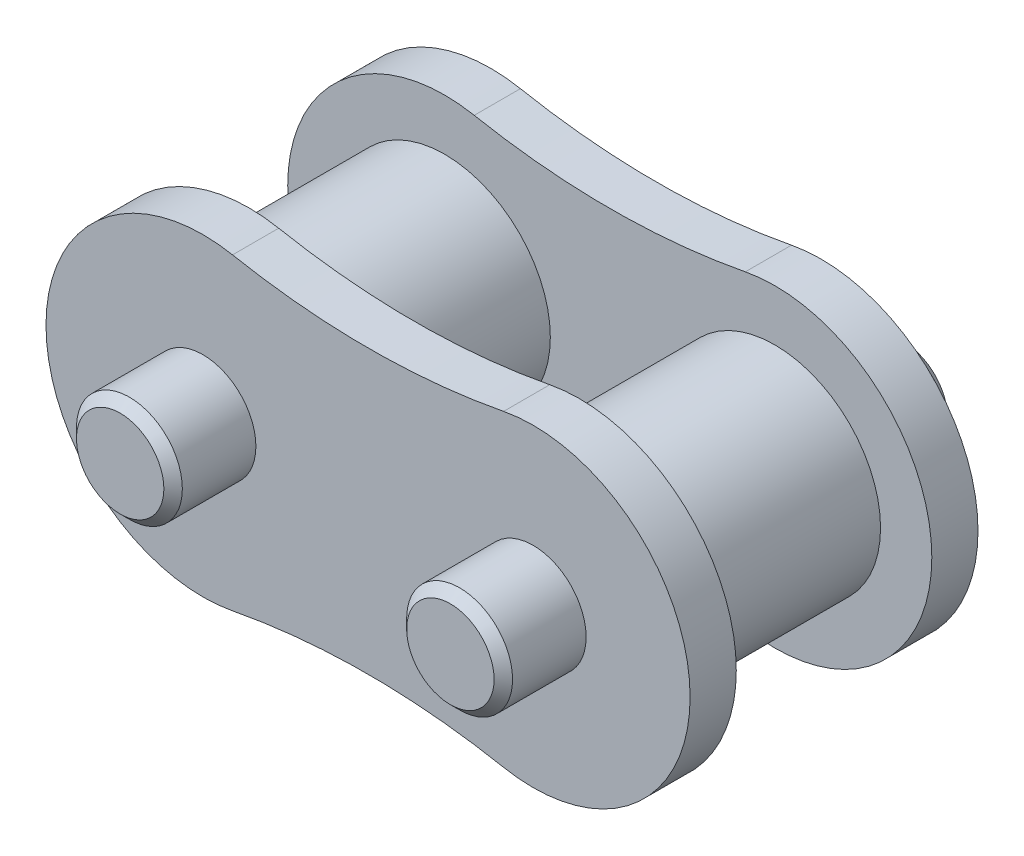
from build123d import *

# Parameters (mm, degrees)
SKETCH_2_R        = 5.08
EXTRUDE_1_DEPTH   = 4.7
EXTRUDE_1_2_DEPTH = 4.7
EXTRUDE_2_DEPTH   = 2.22
SKETCH_4_R        = 2.545
EXTRUDE_3_DEPTH   = 10.9
CHAMFER_1_SIZE    = 0.444


with BuildPart() as part:
    # 草图2 → 拉伸1 (new, symmetric)
    with BuildSketch(Plane.XY):
        with Locations((7.9375, 0)):
            Circle(SKETCH_2_R)
    extrude(amount=EXTRUDE_1_DEPTH, both=True)



with BuildPart() as body_2:
    # 草图2 → Extrude 1 2 (new, symmetric)
    with BuildSketch(Plane.XY):
        with Locations((-7.9375, 0)):
            Circle(SKETCH_2_R)
    extrude(amount=EXTRUDE_1_2_DEPTH, both=True)


with BuildPart() as part_1:
    add(part.part)

    add(body_2.part)  # 拉伸2 merges body 2
    # 草图3 → 拉伸2 (add)
    with BuildSketch(Plane.XY.offset(4.7)):
        with BuildLine():
            ThreePointArc((-6.515962535, 7.409875588), (-15.4825, 0), (-6.515962535, -7.409875588))
            ThreePointArc((-6.515962535, -7.409875588), (0, -6.7905), (6.515962535, -7.409875588))
            ThreePointArc((6.515962535, -7.409875588), (15.4825, 0), (6.515962535, 7.409875588))
            ThreePointArc((6.515962535, 7.409875588), (0, 6.7905), (-6.515962535, 7.409875588))
        make_face()
    extrude_2 = extrude(amount=EXTRUDE_2_DEPTH)

    # 镜向1: 拉伸2 across plane
    add(extrude_2.mirror(Plane.XY))

    # 草图4 → 拉伸3 (add, symmetric)
    with BuildSketch(Plane.XY):
        with Locations((7.9375, 0)):
            Circle(SKETCH_4_R)
        with Locations((-7.9375, 0)):
            Circle(SKETCH_4_R)
    extrude(amount=EXTRUDE_3_DEPTH, both=True)

    # 倒角1
    chamfer_1_edges = [part_1.edges().sort_by_distance(p)[0] for p in [
        (5.3925, 0, -10.9),
        (5.3925, 0, 10.9),
        (-10.4825, 0, -10.9),
        (-10.4825, 0, 10.9),
    ]]
    chamfer(chamfer_1_edges, length=CHAMFER_1_SIZE)


solid = part_1.part
